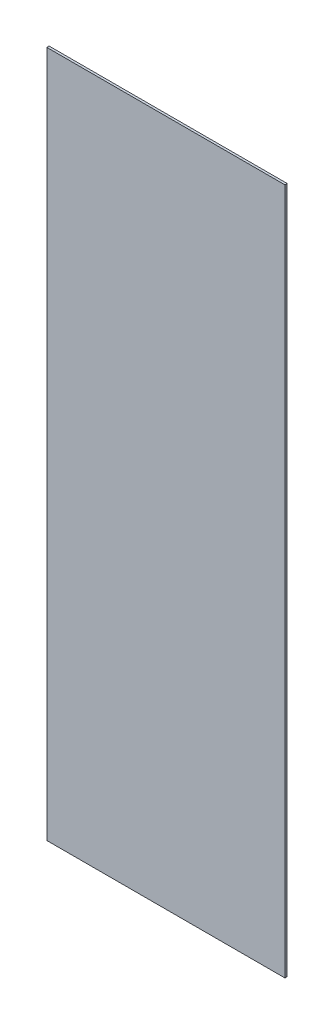
from build123d import *

# Parameters (mm, degrees)
SKETCH_1_W      = 517
SKETCH_1_H      = 1491
EXTRUDE_1_DEPTH = 5


with BuildPart() as part:
    # 草图1 → 凸台-拉伸1 (new body)
    with BuildSketch(Plane.XY):
        Rectangle(SKETCH_1_W, SKETCH_1_H)
    extrude(amount=EXTRUDE_1_DEPTH)


solid = part.part
